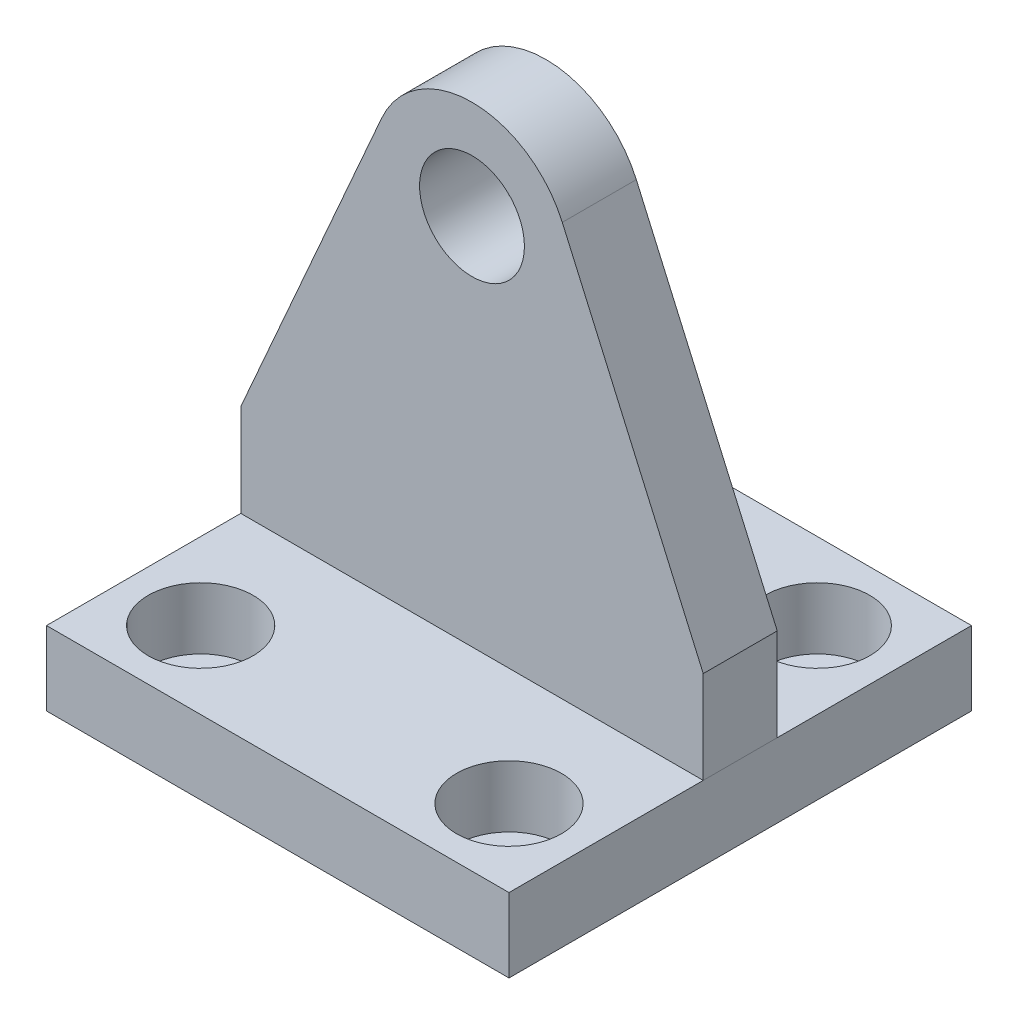
from build123d import *

# Parameters (mm, degrees)
SKETCH1_W                               = 75
SKETCH1_H                               = 75
BOSS_EXTRUDE1_DEPTH                     = 12
SKETCH2_W                               = 75
SKETCH2_H                               = 12
BOSS_EXTRUDE2_DEPTH                     = 76.5
SKETCH3_R                               = 8.5
CUT_EXTRUDE1_DEPTH                      = 106.502369642
CUT_EXTRUDE2_DEPTH                      = 106.502369642
CBORE_FOR_M10_HEX_HEAD_BOLT2_AT_2_COUNT = 2
CBORE_FOR_M10_HEX_HEAD_BOLT2_AT_2_PITCH = 70.710678119
CBORE_FOR_M10_HEX_HEAD_BOLT2_AT_3_COUNT = 2
CBORE_FOR_M10_HEX_HEAD_BOLT2_AT_3_PITCH = 50
CBORE_FOR_M10_HEX_HEAD_BOLT2_AT_4_COUNT = 2
CBORE_FOR_M10_HEX_HEAD_BOLT2_AT_4_PITCH = 50


with BuildPart() as part:
    # Sketch1 → Boss-Extrude1 (new body)
    with BuildSketch(Plane(origin=(0, 0, 0), x_dir=(1, 0, 0), z_dir=(0, 1, 0))):
        Rectangle(SKETCH1_W, SKETCH1_H)
    extrude(amount=BOSS_EXTRUDE1_DEPTH)

    # Sketch6 → CBORE for M10 Hex Head Bolt2 (revolve, cut)
    with BuildSketch(Plane(origin=(25, 12, 25), x_dir=(0, 0, 1), z_dir=(1, 0, 0))):
        Polygon((0, 0), (0, 46.804733405), (5.5, 43.5), (5.5, 10), (8.5, 10), (8.5, 0), align=None)
    cbore_for_m10_hex_head_bolt2 = revolve(axis=Axis((25, 18.35, 25), (0, -1, 0)), mode=Mode.SUBTRACT)

    # CBORE for M10 Hex Head Bolt2 at 2: CBORE for M10 Hex Head Bolt2 ×2
    with Locations(*[Vector(-0.7071067811865476, 0, -0.7071067811865475) * (i * CBORE_FOR_M10_HEX_HEAD_BOLT2_AT_2_PITCH) for i in range(1, CBORE_FOR_M10_HEX_HEAD_BOLT2_AT_2_COUNT)]):
        add(cbore_for_m10_hex_head_bolt2, mode=Mode.SUBTRACT)

    # CBORE for M10 Hex Head Bolt2 at 3: CBORE for M10 Hex Head Bolt2 ×2
    with Locations(*[(-i * CBORE_FOR_M10_HEX_HEAD_BOLT2_AT_3_PITCH, 0, 0) for i in range(1, CBORE_FOR_M10_HEX_HEAD_BOLT2_AT_3_COUNT)]):
        add(cbore_for_m10_hex_head_bolt2, mode=Mode.SUBTRACT)

    # CBORE for M10 Hex Head Bolt2 at 4: CBORE for M10 Hex Head Bolt2 ×2
    with Locations(*[(0, 0, -i * CBORE_FOR_M10_HEX_HEAD_BOLT2_AT_4_PITCH) for i in range(1, CBORE_FOR_M10_HEX_HEAD_BOLT2_AT_4_COUNT)]):
        add(cbore_for_m10_hex_head_bolt2, mode=Mode.SUBTRACT)


with BuildPart() as body_2:
    # Sketch2 → Boss-Extrude2 (new body)
    with BuildSketch(Plane(origin=(0, 12, 0), x_dir=(1, 0, 0), z_dir=(0, 1, 0))):
        Rectangle(SKETCH2_W, SKETCH2_H)
    extrude(amount=BOSS_EXTRUDE2_DEPTH)

    # Sketch3 → Cut-Extrude1 (cut, through all)
    with BuildSketch(Plane.XY.offset(6)):
        with Locations((0, 72.5)):
            Circle(SKETCH3_R)
    extrude(amount=-CUT_EXTRUDE1_DEPTH, mode=Mode.SUBTRACT)

    # Sketch4 → Cut-Extrude2 (cut, through all)
    with BuildSketch(Plane.XY.offset(6)):
        with BuildLine():
            Line((-37.5, 27), (-14.645073815, 78.943742155))
            ThreePointArc((-14.645073815, 78.943742155), (0, 88.5), (14.645073815, 78.943742155))
            Line((14.645073815, 78.943742155), (37.5, 27))
            Line((37.5, 27), (37.5, 88.5))
            Line((37.5, 88.5), (37.5, 96.342049546))
            Line((37.5, 96.342049546), (-37.5, 96.342049546))
            Line((-37.5, 96.342049546), (-37.5, 88.5))
            Line((-37.5, 88.5), (-37.5, 27))
        make_face()
    extrude(amount=-CUT_EXTRUDE2_DEPTH, mode=Mode.SUBTRACT)


solid = Compound([part.part, body_2.part])
